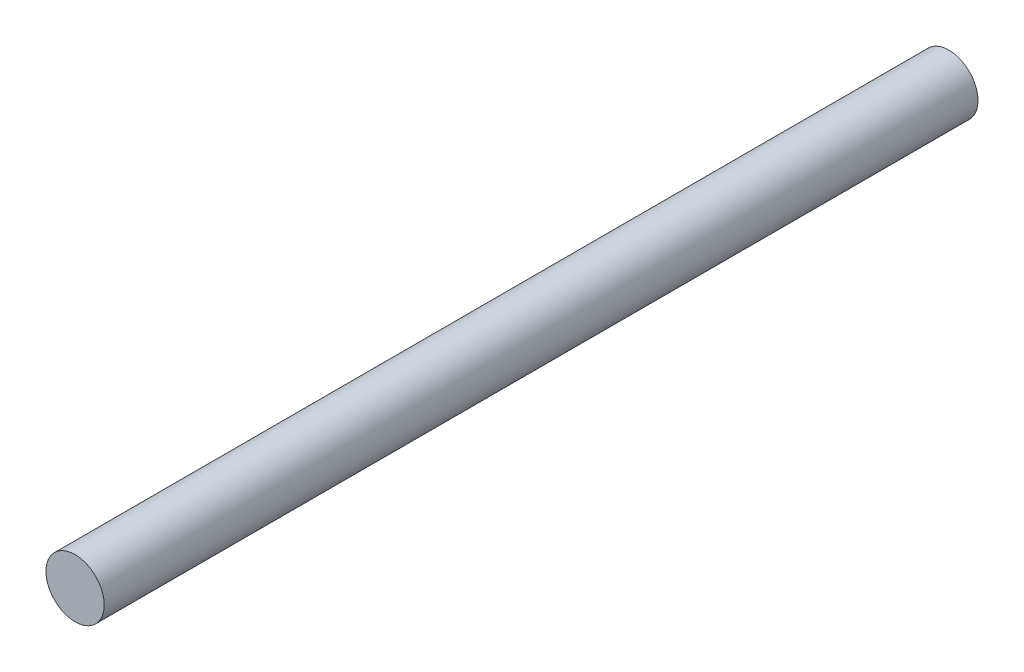
from build123d import *

# Parameters (mm, degrees)
SKETCH1_R           = 1
BOSS_EXTRUDE1_DEPTH = 30


with BuildPart() as part:
    # Sketch1 → Boss-Extrude1 (new body)
    with BuildSketch(Plane.XY):
        Circle(SKETCH1_R)
    extrude(amount=BOSS_EXTRUDE1_DEPTH)


solid = part.part
